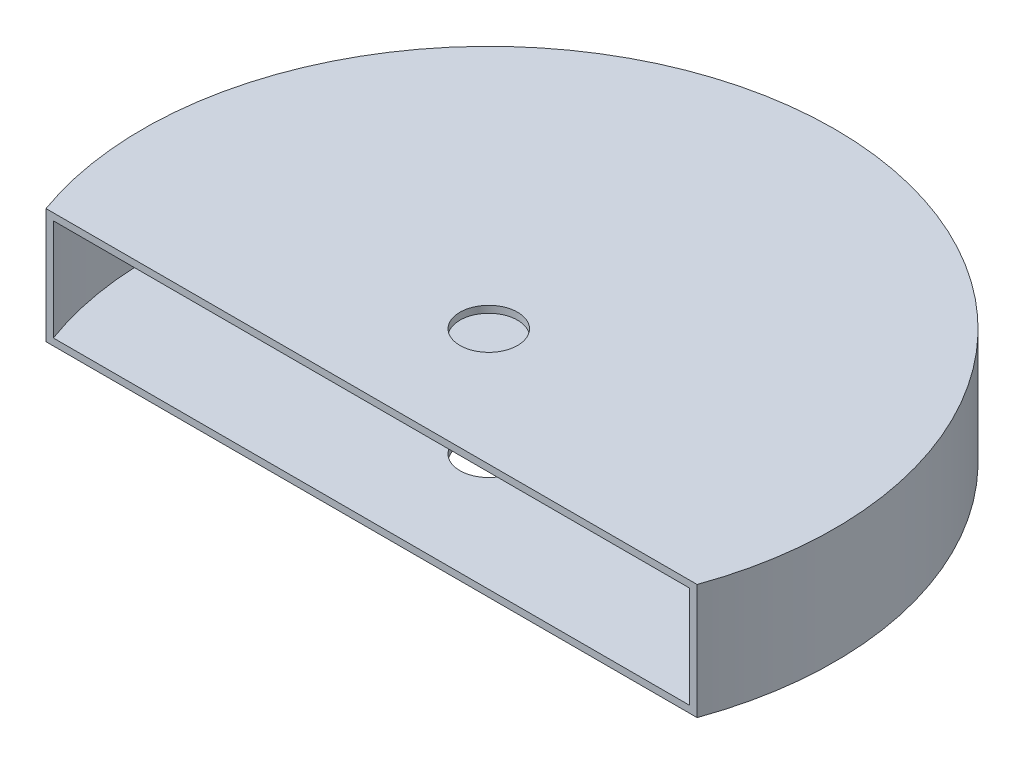
from build123d import *

# Parameters (mm, degrees)
BOSS_EXTRUDE1_DEPTH     = 50
SHELL1_T                = -3
CUT_EXTRUDE1_DEPTH      = 218.944947177
CUT_EXTRUDE1_DEPTH_BACK = 218.944947177
SKETCH2_R               = 12.5


with BuildPart() as part:
    # Sketch1 → Boss-Extrude1 (new body)
    with BuildSketch(Plane(origin=(0, 0, 0), x_dir=(1, 0, 0), z_dir=(0, 1, 0))):
        with BuildLine():
            Line((-141.13085598, -50.814185916), (141.13085598, -50.814185916))
            ThreePointArc((141.13085598, -50.814185916), (0, 150), (-141.13085598, -50.814185916))
        make_face()
    extrude(amount=BOSS_EXTRUDE1_DEPTH)

    # Shell1
    shell1_openings = [part.faces().sort_by_distance(p)[0] for p in [
        (0, 25, 50.814185916),
    ]]
    offset(amount=SHELL1_T, openings=shell1_openings)

    # Sketch2 → Cut-Extrude1 (cut, two sides: drawn at the far end of the back side and taken through both)
    with BuildSketch(Plane(origin=(0, 50, 0), x_dir=(1, 0, 0), z_dir=(0, 1, 0)).offset(-CUT_EXTRUDE1_DEPTH_BACK)):
        with Locations(Location((0, 0, 0), (0, 0, 270))):
            Circle(SKETCH2_R)
    extrude(amount=CUT_EXTRUDE1_DEPTH + CUT_EXTRUDE1_DEPTH_BACK, mode=Mode.SUBTRACT)


solid = part.part
